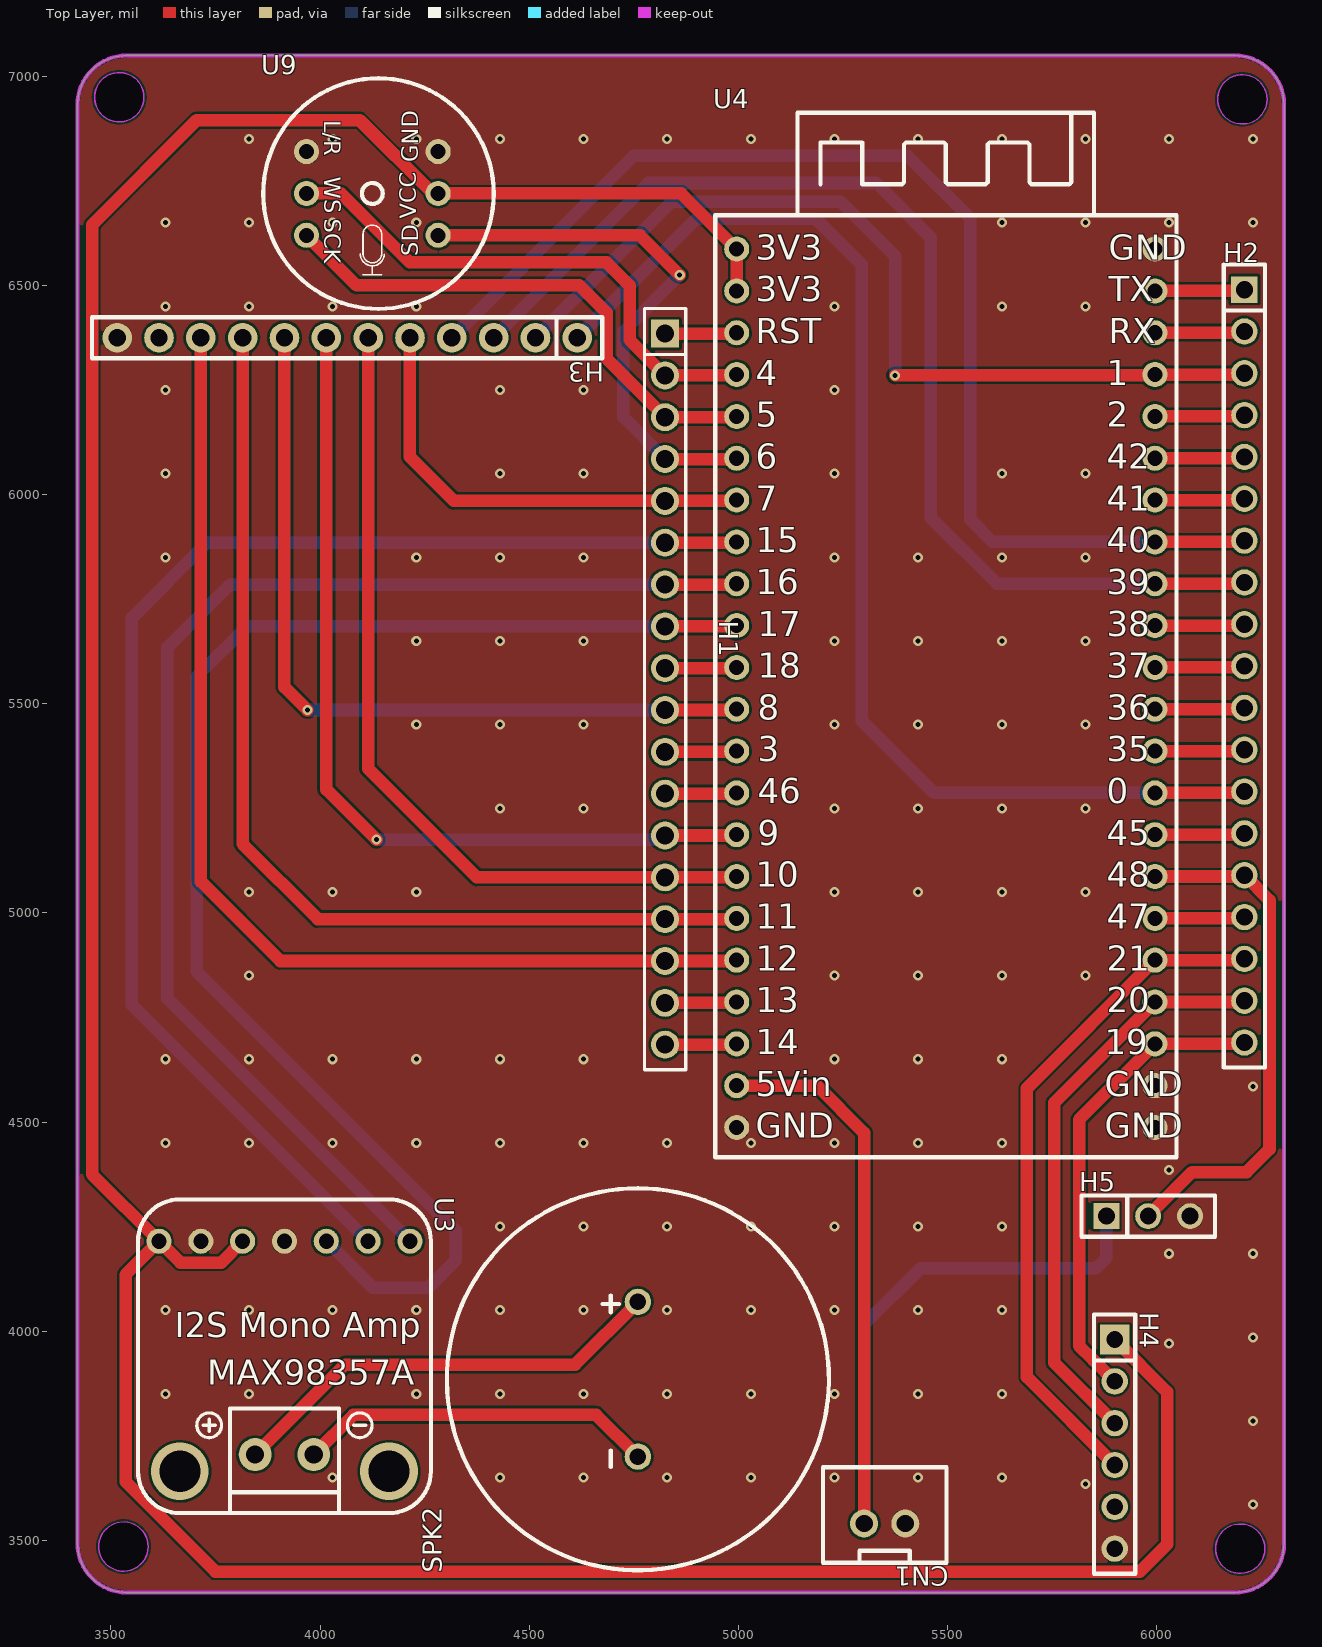
[diagram p0: Top Layer view]
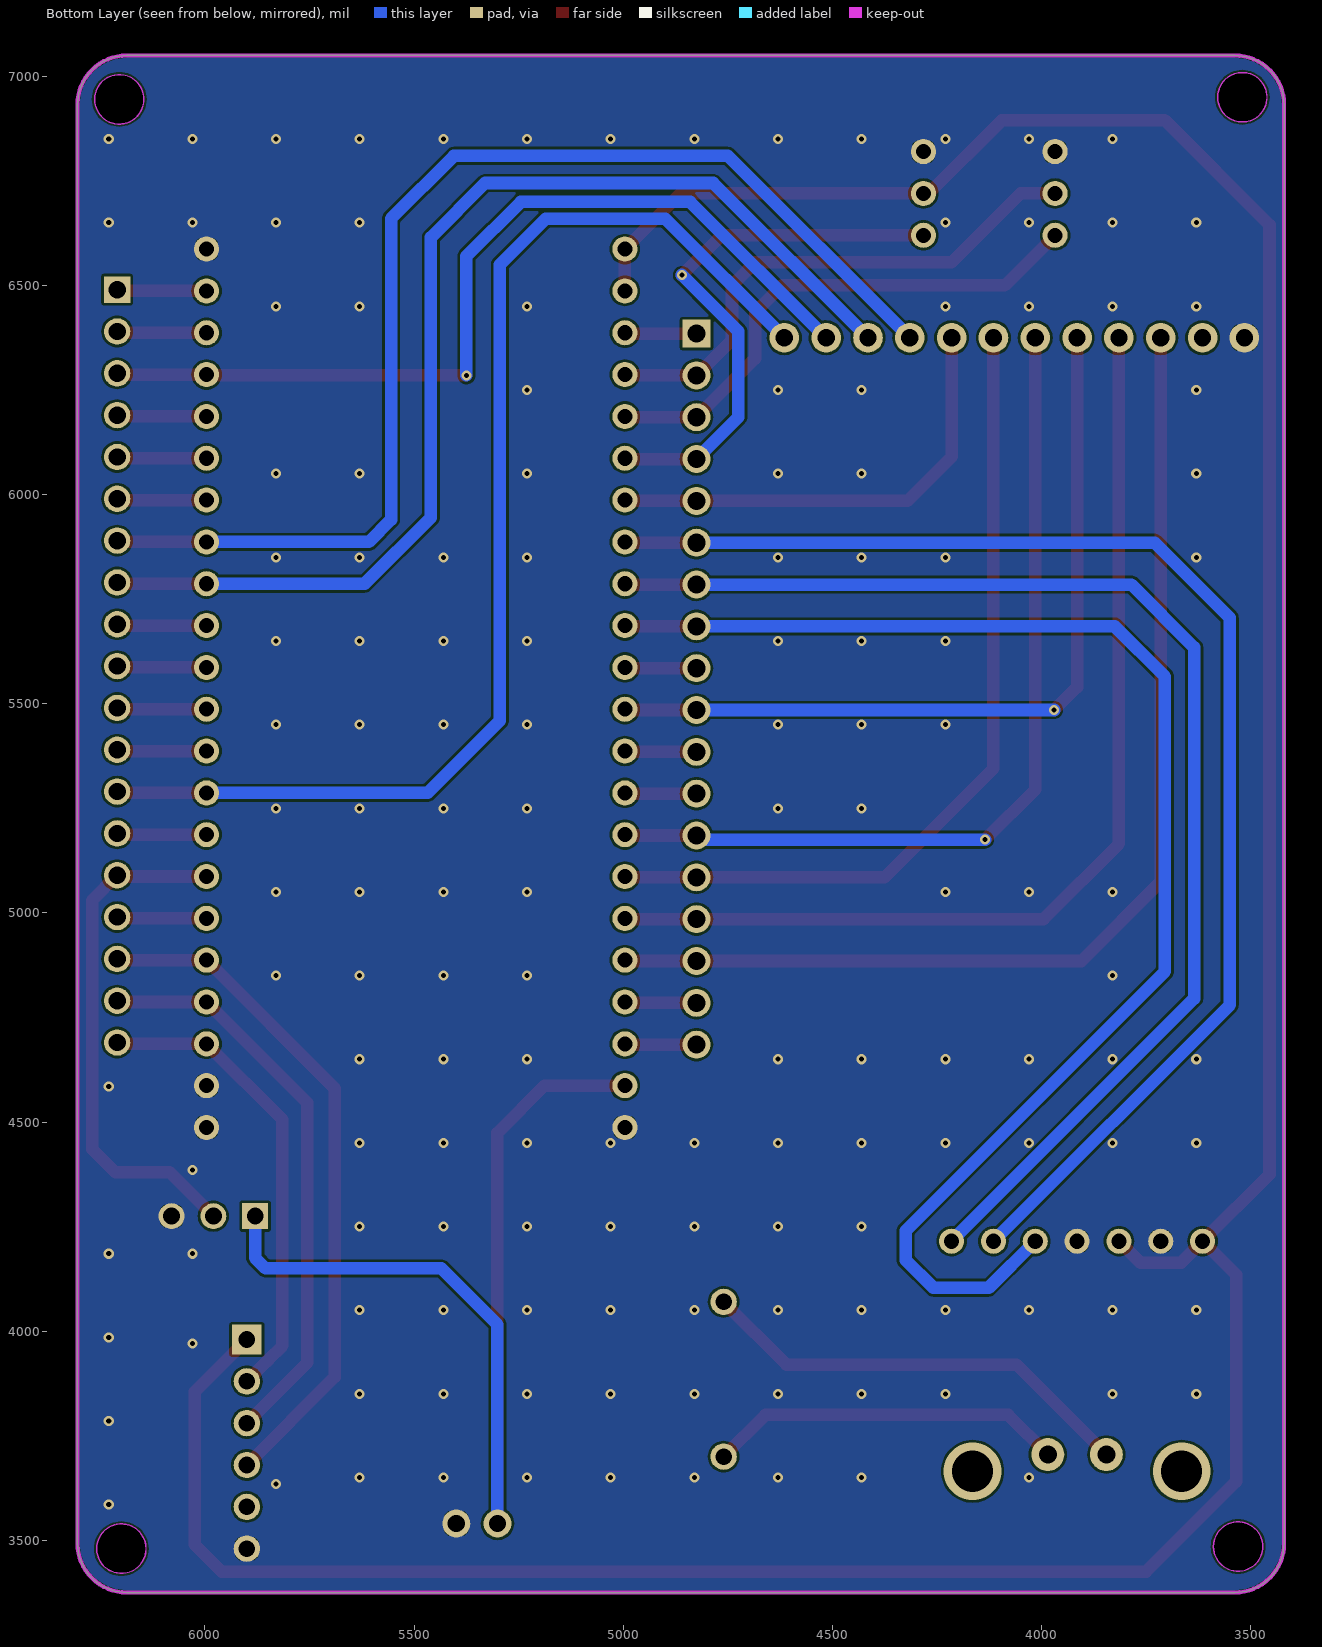
[diagram p1: Bottom Layer view, seen from below]
# Altium PCB MISC52029.pcbdoc
Units mil, origin at the board's own origin, x right, y up, seen from the top; angles counter-clockwise.
Board outline 2885 x 3675 mil, 2 copper layers (Top Layer, Bottom Layer), stack 62.206 mil thick; 10 components, 43 nets, 121 pads, 149 vias.

## Layer stack, top to bottom
Top Solder Mask Layer: solder mask 0.394, Dk 3.3
Top Layer: signal copper 1.379
Dielectric1: surface 59.449, FR4, Dk 4.5
Bottom Layer: signal copper 1.378
Bottom Solder Mask Layer: solder mask 0.394, Dk 3.3

## Board outline
3538.11,7050 ccw(c3538.11,6931.89) 3420,6931.89 3420,3493.11 ccw(c3538.11,3493.11) 3538.11,3375 6186.89,3375 ccw(c6186.89,3493.11) 6305,3493.11 6305,6931.89 ccw(c6186.89,6931.89) 6186.89,7050
cut-out: 6264.06,6945 cw(c6205,6945) 6145.94,6945 cw(c6205,6945)
cut-out: 3579.06,6950 cw(c3520,6950) 3460.94,6950 cw(c3520,6950)
cut-out: 3589.06,3485 cw(c3530,3485) 3470.94,3485 cw(c3530,3485)
cut-out: 6259.06,3480 cw(c6200,3480) 6140.94,3480 cw(c6200,3480)

## Design rules (kind name [scope] priority, off if disabled: settings)
BoardOutlineClearance Plane_Default_1 [All] p2 off: genericclearance=6 ignorepadtopadclearanceinfootprint=FALSE except(0: Arc-SplitContinuation Track-SplitContinuation SMDPad-SplitContinuation THPad-SplitContinuation Via-SplitContinuation Fill-SplitContinuation Region-SplitContinuation Poly-SplitContinuation Text-SplitContinuation Hole-SplitContinuation; 6: Arc-OutlineEdge Track-OutlineEdge SMDPad-OutlineEdge THPad-OutlineEdge Via-OutlineEdge Fill-OutlineEdge Region-OutlineEdge Poly-OutlineEdge Text-OutlineEdge Hole-OutlineEdge Arc-CutoutEdge Track-CutoutEdge SMDPad-CutoutEdge THPad-CutoutEdge Via-CutoutEdge Fill-CutoutEdge Region-CutoutEdge Poly-CutoutEdge Text-CutoutEdge Hole-CutoutEdge)
BoardOutlineClearance Copper_Default_1 [All] p4 off: genericclearance=6 ignorepadtopadclearanceinfootprint=FALSE except(0: Arc-SplitContinuation Track-SplitContinuation SMDPad-SplitContinuation THPad-SplitContinuation Via-SplitContinuation Fill-SplitContinuation Region-SplitContinuation Poly-SplitContinuation Text-SplitContinuation Hole-SplitContinuation; 6: Arc-OutlineEdge Track-OutlineEdge SMDPad-OutlineEdge THPad-OutlineEdge Via-OutlineEdge Fill-OutlineEdge Region-OutlineEdge Poly-OutlineEdge Text-OutlineEdge Hole-OutlineEdge Arc-CutoutEdge Track-CutoutEdge SMDPad-CutoutEdge THPad-CutoutEdge Via-CutoutEdge Fill-CutoutEdge Region-CutoutEdge Poly-CutoutEdge Text-CutoutEdge Hole-CutoutEdge)
BoardOutlineClearance Copper_gge24019_1 [All] p6 off: genericclearance=6 ignorepadtopadclearanceinfootprint=FALSE except(0: Arc-SplitContinuation Track-SplitContinuation SMDPad-SplitContinuation THPad-SplitContinuation Via-SplitContinuation Fill-SplitContinuation Region-SplitContinuation Poly-SplitContinuation Text-SplitContinuation Hole-SplitContinuation; 6: Arc-OutlineEdge Track-OutlineEdge SMDPad-OutlineEdge THPad-OutlineEdge Via-OutlineEdge Fill-OutlineEdge Region-OutlineEdge Text-OutlineEdge Hole-OutlineEdge Arc-CutoutEdge Track-CutoutEdge SMDPad-CutoutEdge THPad-CutoutEdge Via-CutoutEdge Fill-CutoutEdge Region-CutoutEdge Text-CutoutEdge Hole-CutoutEdge; 10: Poly-OutlineEdge Poly-CutoutEdge)
BoardOutlineClearance Default_1 [All] p8: genericclearance=6 ignorepadtopadclearanceinfootprint=FALSE except(0: Arc-SplitContinuation Track-SplitContinuation SMDPad-SplitContinuation THPad-SplitContinuation Via-SplitContinuation Fill-SplitContinuation Region-SplitContinuation Poly-SplitContinuation Text-SplitContinuation Hole-SplitContinuation; 6: Arc-OutlineEdge Track-OutlineEdge SMDPad-OutlineEdge THPad-OutlineEdge Via-OutlineEdge Fill-OutlineEdge Region-OutlineEdge Poly-OutlineEdge Text-OutlineEdge Hole-OutlineEdge Arc-CutoutEdge Track-CutoutEdge SMDPad-CutoutEdge THPad-CutoutEdge Via-CutoutEdge Fill-CutoutEdge Region-CutoutEdge Poly-CutoutEdge Text-CutoutEdge Hole-CutoutEdge)
Clearance Plane_Default [All] p1 off: gap=6 ignorepadtopadclearanceinfootprint=FALSE
Clearance Copper_Default [All] p3 off: gap=6 ignorepadtopadclearanceinfootprint=FALSE
Clearance Copper_gge24019 [All] p5 off: gap=6 ignorepadtopadclearanceinfootprint=FALSE except(10: Poly-Track Poly-SMDPad Poly-THPad Poly-Via Poly-Fill Poly-Region Poly-Poly Poly-Arc Poly-Text Poly-Hole)
Clearance Default [All] p7: gap=6 ignorepadtopadclearanceinfootprint=FALSE
DiffPairsRouting differentialPair [All] p1: maxlimit=6 minlimit=6 mostfreqgap=6 toplayer_minwidth=5 toplayer_prefwidth=10 toplayer_maxwidth=100 toplayer_mingap=6 toplayer_prefgap=6 toplayer_maxgap=6 bottomlayer_minwidth=5 bottomlayer_prefwidth=10 bottomlayer_maxwidth=100 bottomlayer_mingap=6 bottomlayer_prefgap=6 bottomlayer_maxgap=6 maxuncoupledlength=10
HoleToHoleClearance otherClearance [All] p1: gap=11.8 allowstackedmicrovias=TRUE
Length netLength [All] p1: minlimit=0 maxlimit=0
PasteMaskExpansion Common [All] p1: expansion=0
PlaneConnect Default_4 [All] p1: planeconnectstyle=Relief reliefexpansion=20 reliefentries=4 reliefconductorwidth=0 reliefairgap=10
PolygonConnect gge24019 [All] p1 off: connectstyle=Relief reliefconductorwidth=0 reliefentries=4 polygonreliefangle="90 Angle" airgapwidth=1 smdpad.connectstyle=Relief smdpad.reliefconductorwidth=0 smdpad.reliefentries=4 smdpad.polygonreliefangle="90 Angle" smdpad.airgapwidth=10 via.connectstyle=Relief via.reliefconductorwidth=10 via.reliefentries=4 via.polygonreliefangle="90 Angle" via.airgapwidth=10
PolygonConnect Default_5 [All] p2: connectstyle=Relief reliefconductorwidth=0 reliefentries=4 polygonreliefangle="90 Angle" airgapwidth=1 smdpad.connectstyle=Relief smdpad.reliefconductorwidth=0 smdpad.reliefentries=4 smdpad.polygonreliefangle="90 Angle" smdpad.airgapwidth=10 via.connectstyle=Relief via.reliefconductorwidth=10 via.reliefentries=4 via.polygonreliefangle="90 Angle" via.airgapwidth=10
RoutingVias Default_3 [All] p1: holewidth=12 width=24 viastyle="Through Hole" minholewidth=12 minwidth=24 maxholewidth=2362 maxwidth=3938
SolderMaskExpansion Common_1 [IsVia] p1: expansion=-1000 istentingtop=TRUE
SolderMaskExpansion Common_1 [All] p2: expansion=2 istentingtop=FALSE
Width Default_2 [All] p1: maxlimit=1000 minlimit=10 preferedwidth=30

## Components (designator, comment, footprint, x,y, rotation, side; value= is the part's Value field where it differs from the comment)
CN1 "XH2.54*2P_直插" CONN-TH_2P-P2.50-XH2.54-2P 5350,3540 r180 top
H1 "" HDR-TH_18P-P2.54-V-F 4825,5535 r270 top
H2 "C2897382" HDR-TH_19P-P2.54-V-F 6210,5590 r270 top
H3 "" HDR-TH_12P-P2.54-V-F 4065,6375 r180 top
H4 "" HDR-TH_6P-P2.54-V-F 5900,3730 r270 top
H5 "" HDR-TH_3P-P2.54-V-F 5980,4275 r0 top
SPK2 "FS-2308" BEEP-TH_BD23.2-P9.20-D1.0 4760,3885 r90 top
U3 "Adafruit MAX98357 I2S Amp" "MAX98357 I2S AMP MODULE" 3915,4215 r270 top
U4 "NO" ESP32S3 5496.18,5541.93 r0 top
U9 "INMP441" INMP441 4125,6720 r0 top

## Footprints (in the part's own frame and the unit in brackets; to place one, negate y for a bottom-side part, rotate by r counter-clockwise, add the part's x,y. Pads: shape width x height; smd on the part's side, far side on the other; paste and mask are expansions set on the pad)
BEEP-TH_BD23.2-P9.20-D1.0 [mm]
  round 1.6 hole 1: 1(4.7,0) 2(-4.7,0)
  silkscreen extent -11.6,-11.6 11.6,11.6
CONN-TH_2P-P2.50-XH2.54-2P [mm]
  round 1.7 hole 1.05 paste+0 mask+0.05: 1(1.25,0) 2(-1.25,0)
  silkscreen extent -3.75,-3.42 3.75,2.37
ESP32S3 [mil]
  round 60 hole 36: 1(-500,-1055) 2(-500,-955) 3(-500,-855) 4(-500,-755) 5(-500,-655) 6(-500,-555) 7(-500,-455) 8(-500,-355) 9(-500,-255) 10(-500,-155) 11(-500,-55) 12(-500,45) 13(-500,145) 14(-500,245) 15(-500,345) 16(-500,445) 17(-500,545) 18(-500,645) 19(-500,745) 20(-500,845) 21(-500,945) 22(-500,1045) 23(500,-1055) 24(500,-955) 25(500,-855) 26(500,-755) 27(500,-655) 28(500,-555) 29(500,-455) 30(500,-355) 31(500,-255) 32(500,-155) 33(500,-55) 34(500,45) 35(500,145) 36(500,245) 37(500,345) 38(500,445) 39(500,545) 40(500,645) 41(500,745) 42(500,845) 43(500,945) 44(500,1045)
  silkscreen extent -551,-1126 551,1371
HDR-TH_3P-P2.54-V-F [mil]
  rect 62x62 hole 40.16: 1(-100,0)
  round 62 hole 40.16: 2(0,0) 3(100,0)
  silkscreen extent -160,-49 160,49
HDR-TH_6P-P2.54-V-F [mm]
  rect 1.8x1.8 hole 1.02: 1(-6.35,0)
  round 1.6 hole 1.02: 2(-3.81,0) 3(-1.27,0) 4(1.27,0) 5(3.81,0) 6(6.35,0)
  silkscreen extent -7.87,-1.25 7.87,1.25
HDR-TH_12P-P2.54-V-F [mm]
  round 1.8 hole 1.05: 1(-13.97,0) 2(-11.43,0) 3(-8.89,0) 4(-6.35,0) 5(-3.81,0) 6(-1.27,0) 7(1.27,0) 8(3.81,0) 9(6.35,0) 10(8.89,0) 11(11.43,0) 12(13.97,0)
  silkscreen extent -15.49,-1.25 15.49,1.25
HDR-TH_18P-P2.54-V-F [mm]
  rect 1.7x1.7 hole 1.1: 1(-21.59,0)
  round 1.7 hole 1.1: 2(-19.05,0) 3(-16.51,0) 4(-13.97,0) 5(-11.43,0) 6(-8.89,0) 7(-6.35,0) 8(-3.81,0) 9(-1.27,0) 10(1.27,0) 11(3.81,0) 12(6.35,0) 13(8.89,0) 14(11.43,0) 15(13.97,0) 16(16.51,0) 17(19.05,0) 18(21.59,0)
  silkscreen extent -23.11,-1.25 23.11,1.25
HDR-TH_19P-P2.54-V-F [mm]
  rect 1.6x1.6 hole 1.05: 1(-22.86,0)
  round 1.6 hole 1.05: 2(-20.32,0) 3(-17.78,0) 4(-15.24,0) 5(-12.7,0) 6(-10.16,0) 7(-7.62,0) 8(-5.08,0) 9(-2.54,0) 10(0,0) 11(2.54,0) 12(5.08,0) 13(7.62,0) 14(10.16,0) 15(12.7,0) 16(15.24,0) 17(17.78,0) 18(20.32,0) 19(22.86,0)
  silkscreen extent -24.38,-1.25 24.38,1.25
INMP441 [mil]
  round 60 hole 36: 1(157.48,100) 2(157.48,0) 3(157.48,-100) 4(-157.47,100) 5(-157.47,0) 6(-157.47,-100)
  silkscreen extent -261,-276 290,275
"MAX98357 I2S AMP MODULE" [mil]
  round 60 hole 36: 1(0,300) 2(0,200) 3(0,100) 4(0,0) 5(0,-100) 6(0,-200) 7(0,-300)
  round 78.74 hole 43.31 paste+0 mask+4: 8(510,-70) 9(510,70)
  silkscreen extent -100,-350 650,350

## Via types
v1: diameter 24, hole 12, Top Layer to Bottom Layer, 143 vias
v2: diameter 24.02, hole 12, Top Layer to Bottom Layer, 4 vias
v3: diameter 137.8, hole 98.4, Top Layer to Bottom Layer, 2 vias

## Nets (pads, with @x,y where several pads share a name; then routed paths per layer and width w, separated by ;. In a path a pad name is that pad's centre, name@x,y a point inside that pad or via, vN(x,y) a via of type N, cw(c..) or ccw(c..) an arc to the next point about the centre after c; other vN are vias at no path point)
0: H2.13 H3.1 U4.31 | length 2920.3
  Top Layer w30: U4.31 H2.13@6210,5286.93
  Bottom Layer w30: H3.1 4900,6660 5185,6660 5295,6550 5295,5460 5468.07,5286.93 U4.31
1: H2.3 H3.2 U4.41 | length 2169.3
  Top Layer w30: v2(5375,6285) 5994.25,6285 U4.41 H2.3@6210,6286.93
  Bottom Layer w30: H3.2 4840,6700 5245,6700 5375,6570 v2(5375,6285)
2: H2.4 U4.40 | length 213.8
  Top Layer w30: U4.40 H2.4@6210,6186.93
3: H1.11 U4.10 | length 170
  Top Layer w30: H1.11 U4.10@4995,5385
3.3V: H4.1 U3.5 U3.7 U4.21 U4.22 U9.2 | length 8366.8
  Top Layer w30: U3.5 3764,4164 3666,4164 U3.7 ; U4.21 U4.22 4863.11,6720 U9.2 4270,6720 4095,6895 3705,6895 3455,6645 3455,4375 U3.7 ; H4.1 6025,3855 6025,3490 5960,3425 3750,3425 3535,3640 3535,4135 U3.7
4: H1.2 U4.19 U9.5 | length 1283.8
  Top Layer w30: U9.5 4050,6720 4215,6555 4685,6555 4740,6500 4740,6370 H1.2 U4.19@4995,6285
5: H1.3 U4.18 U9.6 | length 1272.1
  Top Layer w30: U9.6 4087.52,6500 4620,6500 4685,6435 4685,6325 H1.3 U4.18@4995,6185
5V-VIN: CN1.1 H5.1 U4.2 | length 2506.5
  Top Layer w30: U4.2 5188.07,4586.93 5300.78,4474.22 CN1.1
  Bottom Layer w30: CN1.1 5300.78,4015.78 5435,4150 5855,4150 5880,4175 H5.1
6: H1.4 U4.17 U9.3 | length 1324.2
  Top Layer w30: U9.3 4765,6620 v2(4860,6525) ; H1.4 U4.17@4995,6085
  Bottom Layer w30: H1.4 4725,6185 4725,6390 v2(4860,6525)
7: H1.5 H3.5 U4.16 | length 1108.5
  Top Layer w30: H3.5 4215,6090 4320,5985 H1.5 U4.16@4995,5985
8: H1.10 H3.8 U4.11 | length 1937.8
  Top Layer w30: H3.8 3915,5540 v2(3970,5485) ; H1.10 U4.11@4995,5485
  Bottom Layer w30: v2(3970,5485) H1.10
9: H1.13 H3.7 U4.8 | length 2113.8
  Top Layer w30: H3.7 4015,5295 v2(4135,5175) ; H1.13 U4.8@4995,5185
  Bottom Layer w30: v2(4135,5175) 4815,5175 H1.13
10: H1.14 H3.6 U4.7 | length 2017.7
  Top Layer w30: H3.6 4115,5345 4375,5085 H1.14 U4.7@4995,5085
11: H1.15 H3.9 U4.6 | length 2464.6
  Top Layer w30: H3.9 3815,5165 3995,4985 H1.15 U4.6@4995,4985
12: H1.16 H3.10 U4.5 | length 2658.7
  Top Layer w30: H3.10 3715,5075 3905,4885 H1.16 U4.5@4995,4885
13: H1.17 U4.4 | length 170
  Top Layer w30: H1.17 U4.4@4995,4785
14: H1.18 U4.3 | length 170
  Top Layer w30: H1.18 U4.3@4995,4685
15: H1.6 U3.2 U4.15 | length 3243.6
  Top Layer w30: H1.6 U4.15@4995,5885
  Bottom Layer w30: U3.2 3550,4780 3550,5705 3730,5885 H1.6
16: H1.7 U3.1 U4.14 | length 3082.4
  Top Layer w30: H1.7 U4.14@4995,5785
  Bottom Layer w30: U3.1 3635,4795 3635,5635 3785,5785 H1.7
17: H1.8 U3.3 U4.13 | length 3375
  Top Layer w30: H1.8 U4.13@4995,5685
  Bottom Layer w30: U3.3 4126.21,4103.79 4258.79,4103.79 4325,4170 4325,4240 3705,4860 3705,5565 3825,5685 H1.8
18: H1.9 U4.12 | length 170
  Top Layer w30: H1.9 U4.12@4995,5585
19: H2.19 H4.2 U4.25 | length 1131.1
  Top Layer w30: H4.2 5852.88,3927.12 cw(c5864.57,3944.57) 5847.12,3932.88 5815,3965 5815,4505.75 U4.25 H2.19@6210,4686.93
20: H2.18 H4.3 U4.26 | length 1380.7
  Top Layer w30: H4.3 5755,3925 5755,4545.75 U4.26 H2.18@6210,4786.93
21: H2.17 H4.4 U4.27 | length 1608.8
  Top Layer w30: H4.4 5690,3890 5690,4580.75 U4.27 ; U4.27@6021.93,4886.93 H2.17@6210,4886.93
35: H2.12 U4.32 | length 213.8
  Top Layer w30: U4.32 H2.12@6210,5386.93
36: H2.11 U4.33 | length 213.8
  Top Layer w30: U4.33 H2.11@6210,5486.93
37: H2.10 U4.34 | length 213.8
  Top Layer w30: U4.34 H2.10@6210,5586.93
38: H2.9 U4.35 | length 213.8
  Top Layer w30: U4.35 H2.9@6210,5686.93
39: H2.8 H3.3 U4.36 | length 2737.6
  Top Layer w30: U4.36 H2.8@6210,5786.93
  Bottom Layer w30: H3.3 4785,6745 5330,6745 5460,6615 5460,5945 5618.07,5786.93 U4.36
40: H2.7 H3.4 U4.37 | length 2879.3
  Top Layer w30: U4.37 H2.7@6210,5886.93
  Bottom Layer w30: H3.4 4750,6810 5405,6810 5555,6660 5555,5940 5608.07,5886.93 U4.37
41: H2.6 U4.38 | length 213.8
  Top Layer w30: U4.38 H2.6@6210,5986.93
42: H2.5 U4.39 | length 213.8
  Top Layer w30: U4.39 H2.5@6210,6086.93
45: H2.14 U4.30 | length 213.8
  Top Layer w30: U4.30 H2.14@6210,5186.93
46: H1.12 U4.9 | length 170
  Top Layer w30: H1.12 U4.9@4995,5285
47: H2.16 U4.28 | length 213.8
  Top Layer w30: U4.28 H2.16@6210,4986.93
48: H2.15 H5.2 U4.29 | length 1249.9
  Top Layer w30: H5.2 6085,4380 6215,4380 6270,4435 6270,5030 H2.15 ; U4.29 H2.15@6210,5086.93
GND: CN1.2 H3.12 H4.6 H5.3 U3.4 U3.6 U4.1 U4.23 U4.24 U4.44 U9.1 U9.4
  other v1: 6230.1,3585.1 5830.1,3635.1 4030.1,3650.1 4430.1,3650.1 4630.1,3650.1 4830.1,3650.1 5030.1,3650.1 5230.1,3650.1 5430.1,3650.1 5630.1,3650.1 6230.1,3785.1 3630.1,3850.1 3830.1,3850.1 4230.1,3850.1 4430.1,3850.1 4630.1,3850.1 4830.1,3850.1 5030.1,3850.1 5230.1,3850.1 5430.1,3850.1 5630.1,3850.1 6030.1,3970.1 6230.1,3985.1 3630.1,4050.1 3830.1,4050.1 4030.1,4050.1 4230.1,4050.1 4430.1,4050.1 4630.1,4050.1 4830.1,4050.1 5030.1,4050.1 5230.1,4050.1 5430.1,4050.1 5630.1,4050.1 6030.1,4185.1 6230.1,4185.1 4430.1,4250.1 4630.1,4250.1 4830.1,4250.1 5030.1,4250.1 5230.1,4250.1 5430.1,4250.1 5630.1,4250.1 6030.1,4385.1 3630.1,4450.1 3830.1,4450.1 4030.1,4450.1 4230.1,4450.1 4430.1,4450.1 4630.1,4450.1 4830.1,4450.1 5030.1,4450.1 5230.1,4450.1 5430.1,4450.1 5630.1,4450.1 6230.1,4585.1 3630.1,4650.1 3830.1,4650.1 4030.1,4650.1 4230.1,4650.1 4430.1,4650.1 4630.1,4650.1 5230.1,4650.1 5430.1,4650.1 5630.1,4650.1 3830.1,4850.1 5230.1,4850.1 5430.1,4850.1 5630.1,4850.1 5830.1,4850.1 3830.1,5050.1 4030.1,5050.1 4230.1,5050.1 5230.1,5050.1 5430.1,5050.1 5630.1,5050.1 5830.1,5050.1 4430.1,5250.1 4630.1,5250.1 5230.1,5250.1 5430.1,5250.1 5630.1,5250.1 5830.1,5250.1 4230.1,5450.1 4430.1,5450.1 4630.1,5450.1 5230.1,5450.1 5430.1,5450.1 5630.1,5450.1 5830.1,5450.1 4230.1,5650.1 4430.1,5650.1 4630.1,5650.1 5230.1,5650.1 5430.1,5650.1 5630.1,5650.1 5830.1,5650.1 3630.1,5850.1 4230.1,5850.1 4430.1,5850.1 4630.1,5850.1 5230.1,5850.1 5430.1,5850.1 5630.1,5850.1 5830.1,5850.1 3630.1,6050.1 4430.1,6050.1 4630.1,6050.1 5230.1,6050.1 5630.1,6050.1 5830.1,6050.1 3630.1,6250.1 4430.1,6250.1 4630.1,6250.1 5230.1,6250.1 3630.1,6450.1 3830.1,6450.1 4030.1,6450.1 4230.1,6450.1 5230.1,6450.1 5630.1,6450.1 5830.1,6450.1 3630.1,6650.1 3830.1,6650.1 4030.1,6650.1 4230.1,6650.1 5630.1,6650.1 5830.1,6650.1 6030.1,6650.1 6230.1,6650.1 3830.1,6850.1 4030.1,6850.1 4230.1,6850.1 4430.1,6850.1 4630.1,6850.1 4830.1,6850.1 5030.1,6850.1 5230.1,6850.1 5430.1,6850.1 5630.1,6850.1 5830.1,6850.1 6030.1,6850.1 6230.1,6850.1
RST: H1.1 U4.20 | length 170
  Top Layer w30: H1.1 U4.20@4995,6385
RX: H2.2 U4.42 | length 213.8
  Top Layer w30: U4.42 H2.2@6210,6386.93
SPEAKER+: SPK2.1 U3.8 | length 1066.2
  Top Layer w30: U3.8 4060,3920 4609.96,3920 SPK2.1
SPEAKER-: SPK2.2 U3.9 | length 855.8
  Top Layer w30: U3.9 4080,3800 4659.96,3800 SPK2.2
TX: H2.1 U4.43 | length 213.8
  Top Layer w30: U4.43 H2.1@6210,6486.93
VCC: H3.11
pads on no net: H4.5
copper on no net:
  other v3: 3665,3665 4165,3665

## Polygon pours and split planes (outlines as drawn)
GND on Top Layer (solid, remove dead copper, pour order 0): 3000,7290 3000,3000 7745,3000 7745,7290
GND on Bottom Layer (solid, remove dead copper, pour order 2): 3215,7290 3215,3270 7590,3270 7590,7290

## Keep-outs
Board Outline Layer:
  region: 6264.06,6945 cw(c6205,6945) 6145.94,6945 cw(c6205,6945)
  circle w0.1: c6205,6945 r59.06
  region: 6264.06,6945 6263.66,6938.14 6262.46,6931.38 6260.49,6924.8 6257.77,6918.5 6254.34,6912.55 6250.24,6907.04 6245.53,6902.04 6240.27,6897.63 6234.53,6893.86 6228.39,6890.77 6221.94,6888.43 6215.25,6886.84 6208.43,6886.04 6201.57,6886.04 6194.75,6886.84 6188.06,6888.43 6181.61,6890.77 6175.47,6893.86 6169.73,6897.63 6164.47,6902.04 6159.76,6907.04 6155.66,6912.55 6152.23,6918.5 6149.51,6924.8 6147.54,6931.38 6146.34,6938.14 6145.94,6945 6146.34,6951.86 6147.54,6958.62 6149.51,6965.2 6152.23,6971.5 6155.66,6977.45 6159.76,6982.96 6164.47,6987.96 6169.73,6992.37 6175.47,6996.14 6181.61,6999.23 6188.06,7001.57 6194.75,7003.16 6201.57,7003.96 6208.43,7003.96 6215.25,7003.16 6221.94,7001.57 6228.39,6999.23 6234.53,6996.14 6240.27,6992.37 6245.53,6987.96 6250.24,6982.96 6254.34,6977.45 6257.77,6971.5 6260.49,6965.2 6262.46,6958.62 6263.66,6951.86
  region: 3579.06,6950 cw(c3520,6950) 3460.94,6950 cw(c3520,6950)
  circle w0.1: c3520,6950 r59.06
  region: 3579.06,6950 3578.66,6943.14 3577.46,6936.38 3575.49,6929.8 3572.77,6923.5 3569.34,6917.55 3565.24,6912.04 3560.53,6907.04 3555.27,6902.63 3549.53,6898.86 3543.39,6895.77 3536.94,6893.43 3530.25,6891.84 3523.43,6891.04 3516.57,6891.04 3509.75,6891.84 3503.06,6893.43 3496.61,6895.77 3490.47,6898.86 3484.73,6902.63 3479.47,6907.04 3474.76,6912.04 3470.66,6917.55 3467.23,6923.5 3464.51,6929.8 3462.54,6936.38 3461.34,6943.14 3460.94,6950 3461.34,6956.86 3462.54,6963.62 3464.51,6970.2 3467.23,6976.5 3470.66,6982.45 3474.76,6987.96 3479.47,6992.96 3484.73,6997.37 3490.47,7001.14 3496.61,7004.23 3503.06,7006.57 3509.75,7008.16 3516.57,7008.96 3523.43,7008.96 3530.25,7008.16 3536.94,7006.57 3543.39,7004.23 3549.53,7001.14 3555.27,6997.37 3560.53,6992.96 3565.24,6987.96 3569.34,6982.45 3572.77,6976.5 3575.49,6970.2 3577.46,6963.62 3578.66,6956.86
  region: 3589.06,3485 cw(c3530,3485) 3470.94,3485 cw(c3530,3485)
  circle w0.1: c3530,3485 r59.06
  region: 3589.06,3485 3588.66,3478.14 3587.46,3471.38 3585.49,3464.8 3582.77,3458.5 3579.34,3452.55 3575.24,3447.04 3570.53,3442.04 3565.27,3437.63 3559.53,3433.86 3553.39,3430.77 3546.94,3428.43 3540.25,3426.84 3533.43,3426.04 3526.57,3426.04 3519.75,3426.84 3513.06,3428.43 3506.61,3430.77 3500.47,3433.86 3494.73,3437.63 3489.47,3442.04 3484.76,3447.04 3480.66,3452.55 3477.23,3458.5 3474.51,3464.8 3472.54,3471.38 3471.34,3478.14 3470.94,3485 3471.34,3491.86 3472.54,3498.62 3474.51,3505.2 3477.23,3511.5 3480.66,3517.45 3484.76,3522.96 3489.47,3527.96 3494.73,3532.37 3500.47,3536.14 3506.61,3539.23 3513.06,3541.57 3519.75,3543.16 3526.57,3543.96 3533.43,3543.96 3540.25,3543.16 3546.94,3541.57 3553.39,3539.23 3559.53,3536.14 3565.27,3532.37 3570.53,3527.96 3575.24,3522.96 3579.34,3517.45 3582.77,3511.5 3585.49,3505.2 3587.46,3498.62 3588.66,3491.86
  region: 6259.06,3480 cw(c6200,3480) 6140.94,3480 cw(c6200,3480)
  circle w0.1: c6200,3480 r59.06
  region: 6259.06,3480 6258.66,3473.14 6257.46,3466.38 6255.49,3459.8 6252.77,3453.5 6249.34,3447.55 6245.24,3442.04 6240.53,3437.04 6235.27,3432.63 6229.53,3428.86 6223.39,3425.77 6216.94,3423.43 6210.25,3421.84 6203.43,3421.04 6196.57,3421.04 6189.75,3421.84 6183.06,3423.43 6176.61,3425.77 6170.47,3428.86 6164.73,3432.63 6159.47,3437.04 6154.76,3442.04 6150.66,3447.55 6147.23,3453.5 6144.51,3459.8 6142.54,3466.38 6141.34,3473.14 6140.94,3480 6141.34,3486.86 6142.54,3493.62 6144.51,3500.2 6147.23,3506.5 6150.66,3512.45 6154.76,3517.96 6159.47,3522.96 6164.73,3527.37 6170.47,3531.14 6176.61,3534.23 6183.06,3536.57 6189.75,3538.16 6196.57,3538.96 6203.43,3538.96 6210.25,3538.16 6216.94,3536.57 6223.39,3534.23 6229.53,3531.14 6235.27,3527.37 6240.53,3522.96 6245.24,3517.96 6249.34,3512.45 6252.77,3506.5 6255.49,3500.2 6257.46,3493.62 6258.66,3486.86
  lines w10: 3420,3493.11 3420,6931.89 cw(c3538.11,6931.89) 3538.11,7050 6186.89,7050 cw(c6186.89,6931.89) 6305,6931.89 6305,3493.11 cw(c6186.89,3493.11) 6186.89,3375 3538.11,3375 cw(c3538.11,3493.11) 3420,3493.11

## Silkscreen, mask and mechanical layers (free items; w line width, h text height)
Mechanical Layer:
  circle w0.1: c6205,6945 r59.06
  circle w0.1: c3520,6950 r59.06
  circle w0.1: c3530,3485 r59.06
  circle w0.1: c6200,3480 r59.06